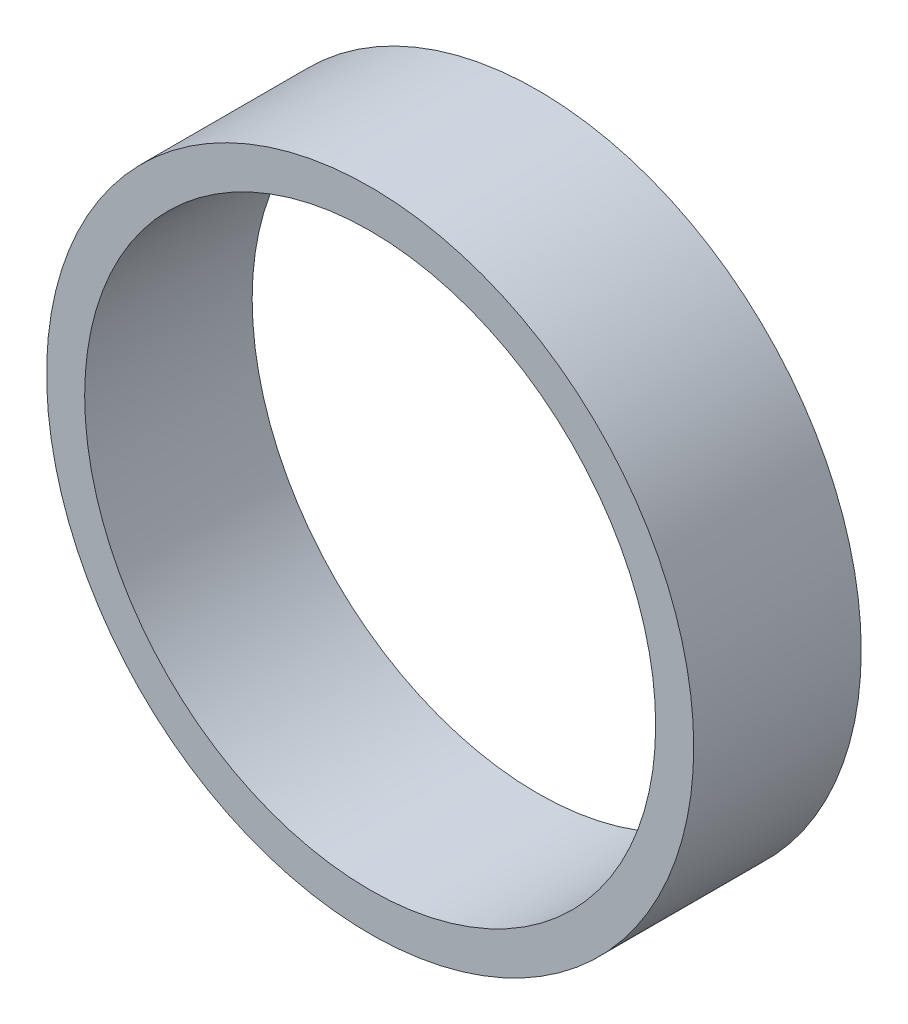
from build123d import *

# Parameters (mm, degrees)
SKETCH_1_R      = 42.5
SKETCH_1_R_2    = 37.5
EXTRUDE_1_DEPTH = 22


with BuildPart() as part:
    # 草图1 → 凸台-拉伸1 (new body)
    with BuildSketch(Plane.XY):
        Circle(SKETCH_1_R)
        Circle(SKETCH_1_R_2, mode=Mode.SUBTRACT)
    extrude(amount=EXTRUDE_1_DEPTH)


solid = part.part
